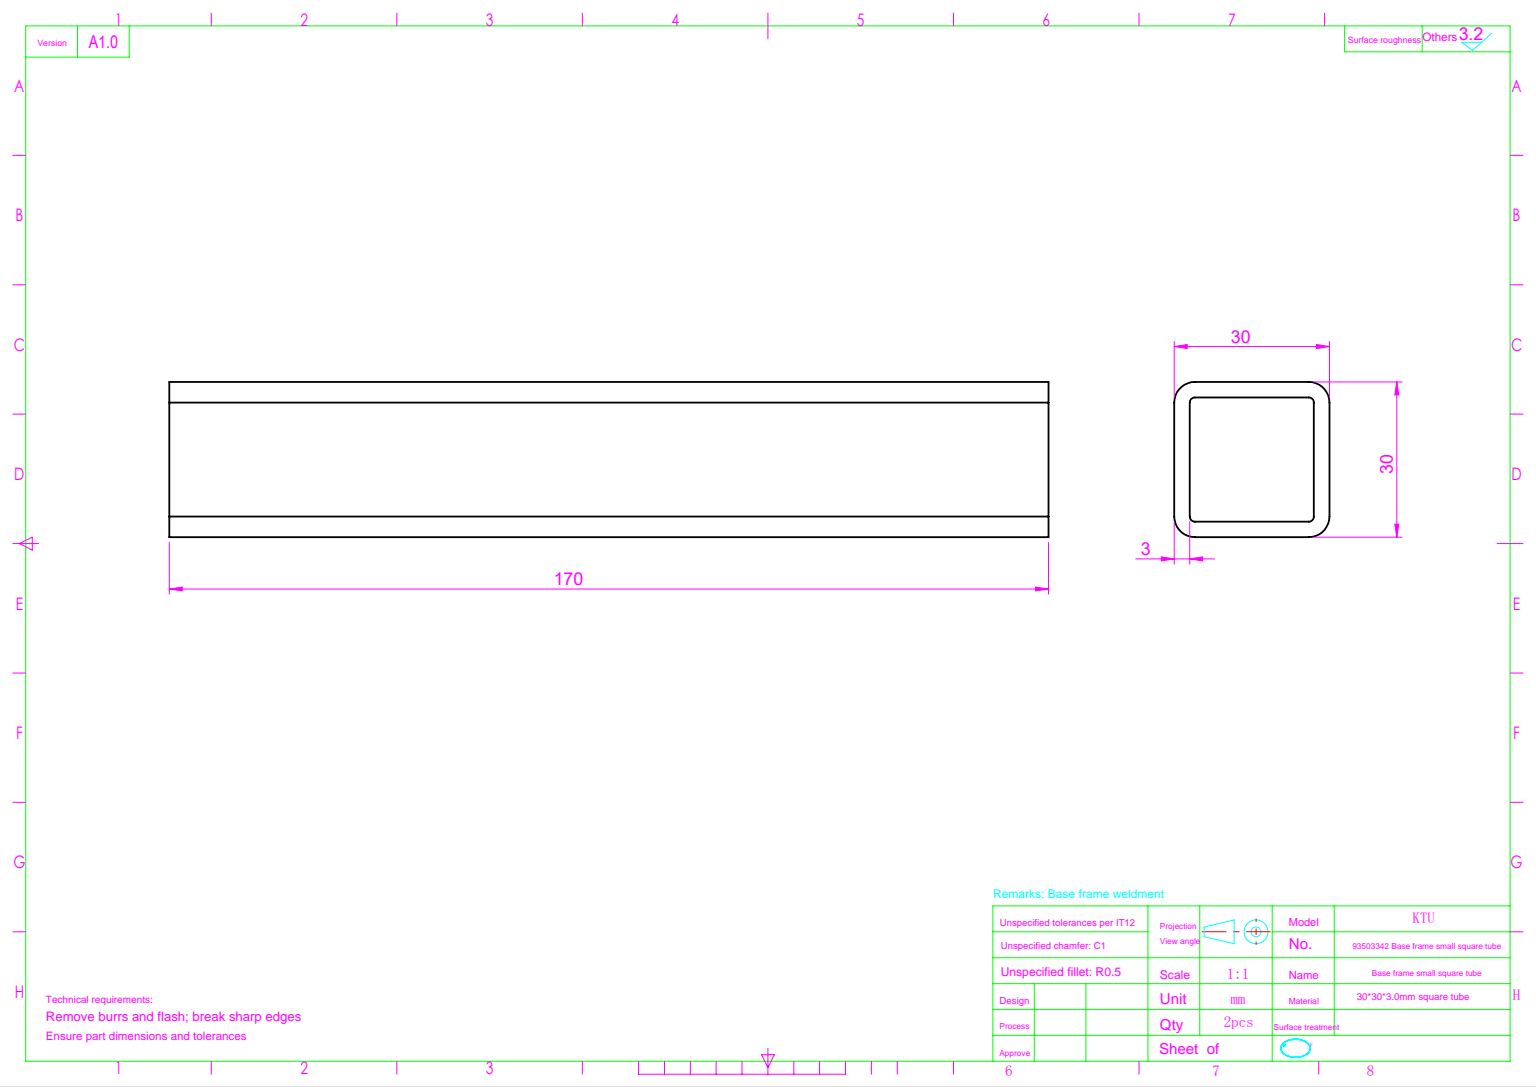
SolidWorks part; units mm, degrees
ref_plane "前视基准面" through (0, 0, 0) normal (0, 0, 1) x (1, 0, 0)
ref_plane "上视基准面" through (0, 0, 0) normal (0, 1, 0) x (1, 0, 0)
ref_plane "右视基准面" through (0, 0, 0) normal (1, 0, 0) x (0, 0, -1)
sketch "草图2" plane through (0, 0, 0) normal (0, 0, 1) x (1, 0, 0)
  line L1 (-11, 15) -> (11, 15)
  line L2 (-15, 11) -> (-15, -11)
  line L3 (-11, -15) -> (11, -15)
  line L4 (15, 11) -> (15, -11)
  line L5 (-15, 15) -> (15, -15) construction
  line L6 (-15, -15) -> (15, 15) construction
  arc A0 (11, 15) -> (15, 11) centre (11, 11) cw
  arc A1 (11, -15) -> (15, -11) centre (11, -11) ccw
  arc A2 (-15, -11) -> (-11, -15) centre (-11, -11) ccw
  arc A3 (-11, 15) -> (-15, 11) centre (-11, 11) ccw
  point P0 (0, 0)
  dimension "D3" = 4
  dimension "D1" = 30
  dimension "D2" = 30
extrude "拉伸-薄壁1" add sketch "草图2" along normal mid plane 170 thin
